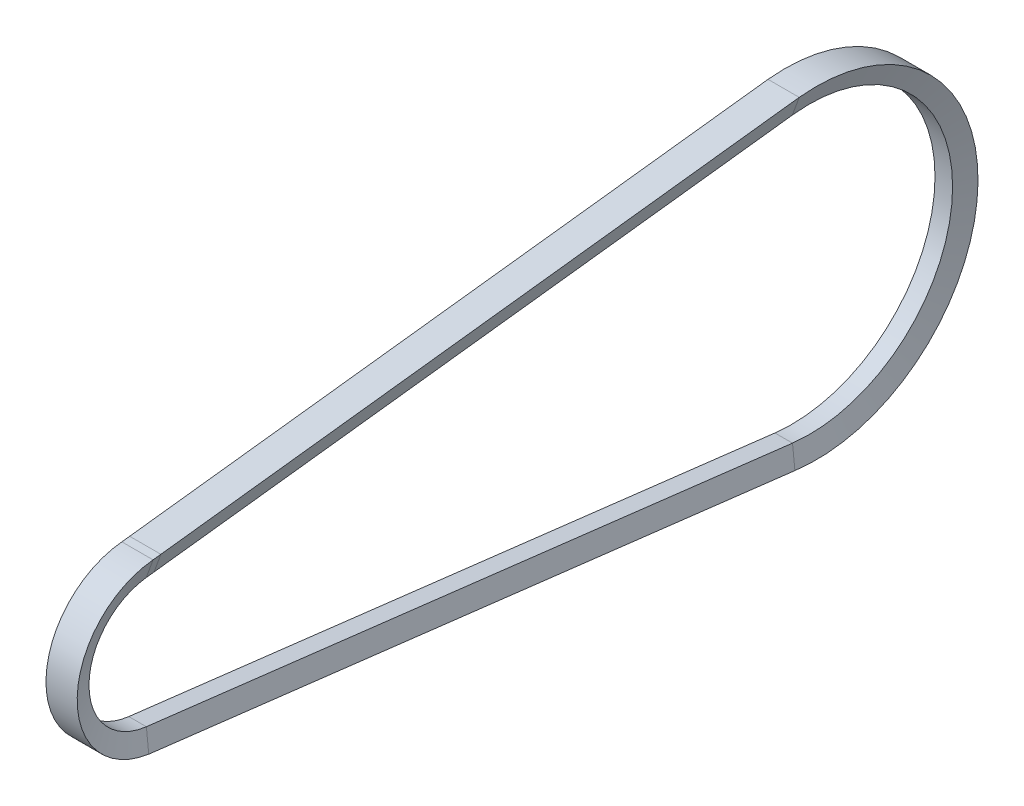
from build123d import *


with BuildPart() as part:
    # Sweep1: sweep along a path in Sketch3
    with BuildLine(Plane(origin=(0, 0, 0), x_dir=(0, 0, -1), z_dir=(1, 0, 0))) as sweep1_path:
        Line((-2.5, -0.149340538), (204.523809524, 24.672873107))
        ThreePointArc((204.523809524, 24.672873107), (256, -21), (204.523809524, -66.672873107))
        Line((204.523809524, -66.672873107), (-2.5, -41.850659462))
        ThreePointArc((-2.5, -41.850659462), (-21, -21), (-2.5, -0.149340538))
    # Sketch2 → Sweep1 (sweep)
    with BuildSketch(Plane.XY):
        Polygon((-5, 6), (5, 6), (2.816178594, 0), (-2.816178594, 0), align=None)
    sweep(path=sweep1_path.line)


solid = part.part
